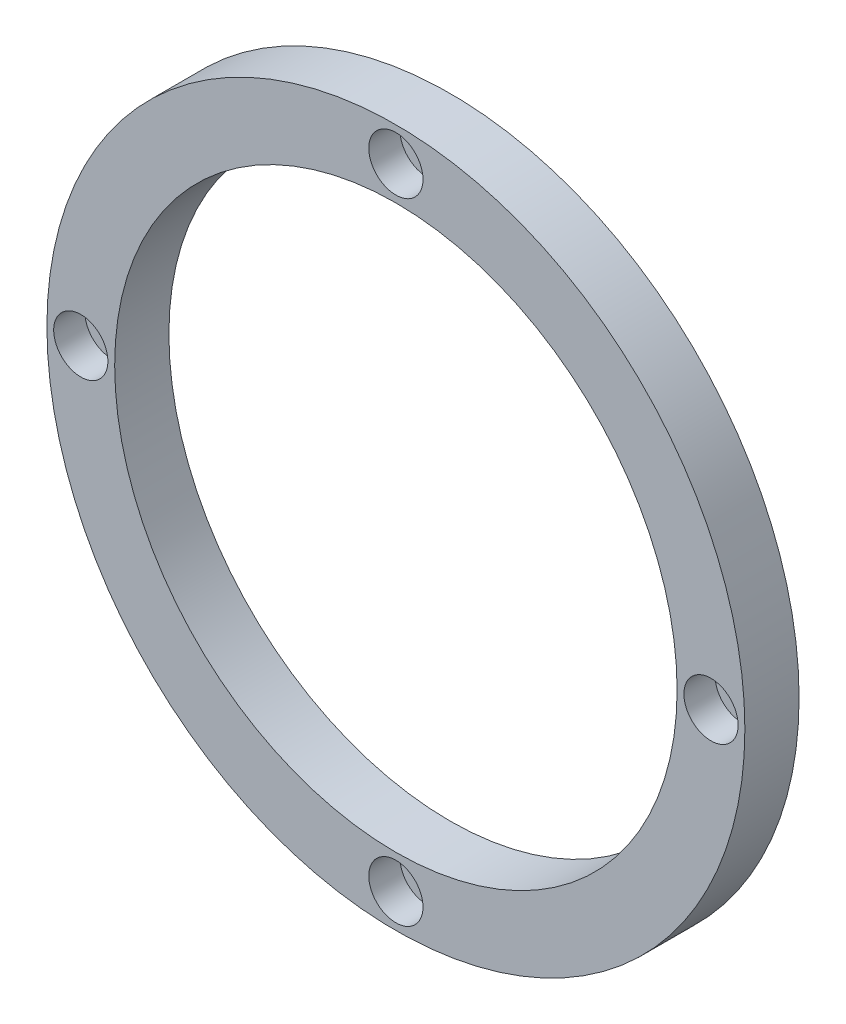
SolidWorks part; units mm, degrees
ref_plane "Front Plane" through (0, 0, 0) normal (0, 0, 1) x (1, 0, 0)
ref_plane "Top Plane" through (0, 0, 0) normal (0, 1, 0) x (1, 0, 0)
ref_plane "Right Plane" through (0, 0, 0) normal (1, 0, 0) x (0, 0, -1)
sketch "Sketch1" plane through (0, 0, 0) normal (0, 0, 1) x (1, 0, 0)
  circle A0 centre (0, 0) radius 41.5
  circle A1 centre (0, 0) radius 51.5
  dimension "D1" = 103
  dimension "D2" = 83
extrude "Boss-Extrude1" add sketch "Sketch1" along normal blind 8
hole_wizard "Hole size per hex socket cap screw type1" positions "Sketch4" profile "Sketch5" counterbore size "M4" standard "GB"
sketch "Sketch4" plane through (0, 0, 8) normal (0, 0, 1) x (1, 0, 0)
  circle A0 centre (0, 0) radius 46.5 construction
  point P0 (0, 46.5)
  dimension "D1" = 93
sketch "Sketch5" plane through (0, 46.5, 8) normal (1, 0, 0) x (0, -1, 0)
  line L0 (0, 0) -> (0, 18.3519)
  line L1 (0, 18.3519) -> (2.25, 17)
  line L2 (2.25, 17) -> (2.25, 4.6)
  line L3 (2.25, 4.6) -> (4, 4.6)
  line L4 (4, 4.6) -> (4, 0)
  line L5 (4, 0) -> (0, 0)
  line L10 (0, 18.3519) -> (-2.25, 17) construction
  line L11 (0, -6.35) -> (0, 107.95) construction
  dimension "孔直径" = 4.5
  dimension "孔深度" = 17
  dimension "柱形沉头孔直径" = 8
  dimension "柱形沉头孔深度" = 4.6
  dimension "导头角度" = 118
pattern_circular "CirPattern1" count 4 over 360 about axis through (0, 0, 0) along (0, 0, 1) of "Hole size per hex socket cap screw type1"
